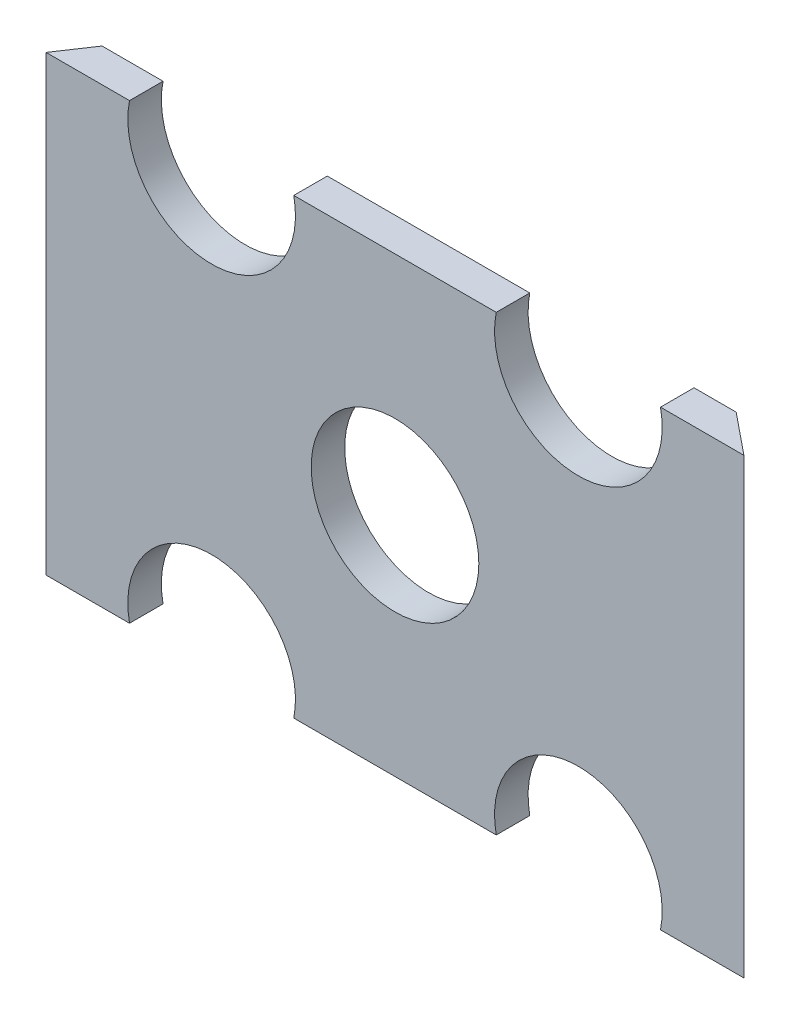
SolidWorks part; units mm, degrees
ref_plane "Front Plane" through (0, 0, 0) normal (0, 0, 1) x (1, 0, 0)
ref_plane "Top Plane" through (0, 0, 0) normal (0, 1, 0) x (1, 0, 0)
ref_plane "Right Plane" through (0, 0, 0) normal (1, 0, 0) x (0, 0, -1)
sketch "Sketch1" plane through (0, 0, 0) normal (0, 0, 1) x (1, 0, 0)
  line L0 (166.5, 216) -> (166.5, -55.6169) construction
  line L1 (0, 0) -> (39.8082, 0)
  line L2 (0, 0) -> (0, 216)
  line L3 (0, 216) -> (39.8082, 216)
  line L4 (333, 0) -> (333, 216)
  line L5 (0, 108) -> (352.8795, 108) construction
  line L6 (79, 275.4091) -> (79, -111.6998) construction
  line L7 (254, 284.9842) -> (254, -95.2853) construction
  line L8 (-14.3952, 208) -> (414.4339, 208) construction
  line L9 (-34.2294, 8) -> (352.8795, 8) construction
  line L10 (118.1918, 216) -> (214.8082, 216)
  line L11 (293.1918, 216) -> (333, 216)
  line L12 (118.1918, 0) -> (214.8082, 0)
  line L13 (293.1918, 0) -> (333, 0)
  circle A0 centre (166.5, 108) radius 40
  arc A1 (214.8082, 216) -> (293.1918, 216) centre (254, 208) ccw
  arc A2 (293.1918, 0) -> (214.8082, 0) centre (254, 8) ccw
  arc A3 (118.1918, 0) -> (39.8082, 0) centre (79, 8) ccw
  arc A4 (39.8082, 216) -> (118.1918, 216) centre (79, 208) ccw
  dimension "D7" = 80
  dimension "D8" = 80
  dimension "D9" = 80
  dimension "D10" = 80
  dimension "D11" = 80
  dimension "D1" = 216
  dimension "D2" = 333
  dimension "D3" = 100
  dimension "D4" = 100
  dimension "D5" = 87.5
  dimension "D6" = 87.5
  dimension "D12" = 166.5
extrude "Boss-Extrude1" add sketch "Sketch1" along normal blind 16
sketch "Sketch2" plane through (0, 0, 0) normal (0, -1, 0) x (1, 0, 0)
  line L0 (0, 16) -> (10.7, 0)
  line L1 (0, 0) -> (39.8082, 0) construction
  line L2 (333, 16) -> (313.3, 0)
  line L3 (293.1918, 0) -> (333, 0) construction
  line L4 (0, 16) -> (0, 0) construction
  line L5 (0, 16) -> (0, 0)
  line L6 (333, 16) -> (333, 0) construction
  line L7 (0, 0) -> (10.7, 0)
  line L8 (333, 16) -> (333, 0)
  line L9 (313.3, 0) -> (333, 0)
  dimension "D1" = 19.7
  dimension "D2" = 10.7
extrude "Cut-Extrude1" cut sketch "Sketch2" against normal through all
